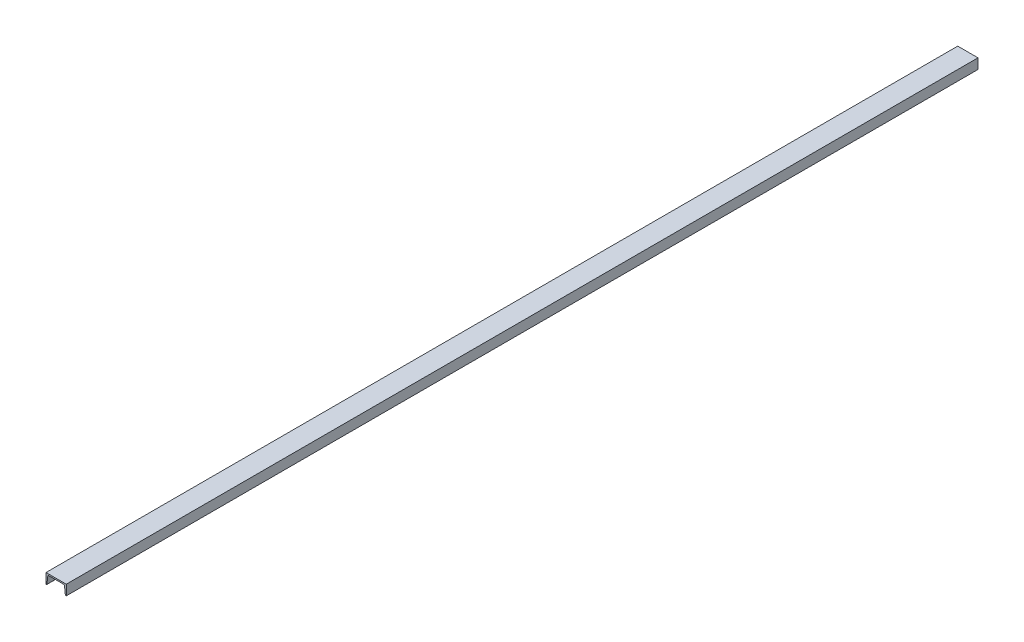
from build123d import *

# Parameters (mm, degrees)
BOSS_EXTRUDE1_DEPTH = 4500


with BuildPart() as part:
    # Sketch1 → Boss-Extrude1 (new body)
    with BuildSketch(Plane.XY):
        with BuildLine():
            Line((0, 0), (0, 50))
            Line((0, 50), (100, 50))
            Line((100, 50), (100, 0))
            Line((100, 0), (97.451472673, 0))
            ThreePointArc((97.451472673, 0), (96.119850629, 0.507759157), (95.464371872, 1.773217267))
            Line((95.464371872, 1.773217267), (91.247290138, 38.723854473))
            ThreePointArc((91.247290138, 38.723854473), (89.608593246, 41.887499748), (86.279538137, 43.156897641))
            Line((86.279538137, 43.156897641), (13.720461863, 43.156897641))
            ThreePointArc((13.720461863, 43.156897641), (10.391406754, 41.887499748), (8.752709862, 38.723854473))
            Line((8.752709862, 38.723854473), (4.535628128, 1.773217267))
            ThreePointArc((4.535628128, 1.773217267), (3.880149371, 0.507759157), (2.548527327, 0))
            Line((2.548527327, 0), (0, 0))
        make_face()
    extrude(amount=BOSS_EXTRUDE1_DEPTH)


solid = part.part
